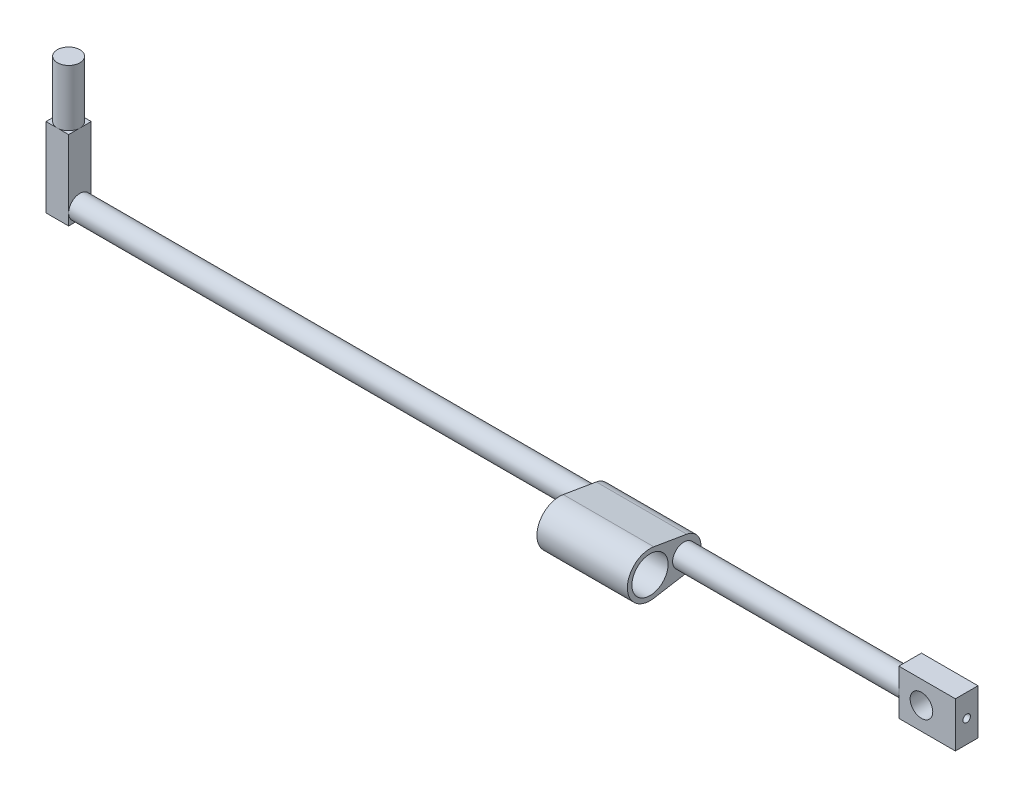
from build123d import *

# Parameters (mm, degrees)
SKETCH_6_W             = 25
SKETCH_6_H             = 20
SKETCH_6_R             = 5
EXTRUDE_4_DEPTH        = 10
SKETCH_7_R             = 5
EXTRUDE_5_DEPTH        = 367
HOLE_WIZARD_M4_1_D     = 3.3
HOLE_WIZARD_M4_1_DEPTH = 5
HOLE_WIZARD_M4_1_TIP   = 0.991420021
EXTRUDE_6_DEPTH        = 10
SKETCH_11_R            = 5
EXTRUDE_7_DEPTH        = 25
SKETCH_12_R            = 8
EXTRUDE_8_DEPTH        = 40


with BuildPart() as part:
    # 草图6 → 凸台-拉伸4 (new body)
    with BuildSketch(Plane.XY):
        with Locations((12.5, 10)):
            Rectangle(SKETCH_6_W, SKETCH_6_H)
        with Locations((10, 10)):
            Circle(SKETCH_6_R, mode=Mode.SUBTRACT)
    extrude(amount=EXTRUDE_4_DEPTH)

    # 草图7 → 凸台-拉伸5 (add)
    with BuildSketch(Plane.ZY):
        with Locations((5, 10)):
            Circle(SKETCH_7_R)
    extrude(amount=EXTRUDE_5_DEPTH)

    # M4 螺纹孔1
    with Locations(Plane(origin=(25, 0, 0), x_dir=(0, 0, -1), z_dir=(1, 0, 0))):
        with Locations((-5, 10)):
            Hole(HOLE_WIZARD_M4_1_D / 2, depth=HOLE_WIZARD_M4_1_DEPTH)
            with Locations((0, 0, -(HOLE_WIZARD_M4_1_DEPTH + HOLE_WIZARD_M4_1_TIP / 2))):  # 118° drill point
                Cone(0, HOLE_WIZARD_M4_1_D / 2, HOLE_WIZARD_M4_1_TIP, mode=Mode.SUBTRACT)

    # 草图10 → 凸台-拉伸6 (add)
    with BuildSketch(Plane.ZY.offset(367)):
        Polygon((0, 40), (10, 40), (10, 5), (0, 5), (0, 15), align=None)
    extrude(amount=EXTRUDE_6_DEPTH)

    # 草图11 → 凸台-拉伸7 (add)
    with BuildSketch(Plane(origin=(0, 40, 0), x_dir=(1, 0, 0), z_dir=(0, 1, 0))):
        with Locations(Location((-372, -5, 0), (0, 0, 270))):
            Circle(SKETCH_11_R)
    extrude(amount=EXTRUDE_7_DEPTH)

    # 草图12 → 凸台-拉伸8 (add)
    with BuildSketch(Plane.ZY.offset(100)):
        with BuildLine():
            Line((3.75, 17.395099729), (18.333333333, 19.860132972))
            ThreePointArc((18.333333333, 19.860132972), (30, 10), (18.333333333, 0.139867028))
            Line((18.333333333, 0.139867028), (3.75, 2.604900271))
            ThreePointArc((3.75, 2.604900271), (-2.5, 10), (3.75, 17.395099729))
        make_face()
        with Locations((20, 10)):
            Circle(SKETCH_12_R, mode=Mode.SUBTRACT)
    extrude(amount=EXTRUDE_8_DEPTH)


solid = part.part
